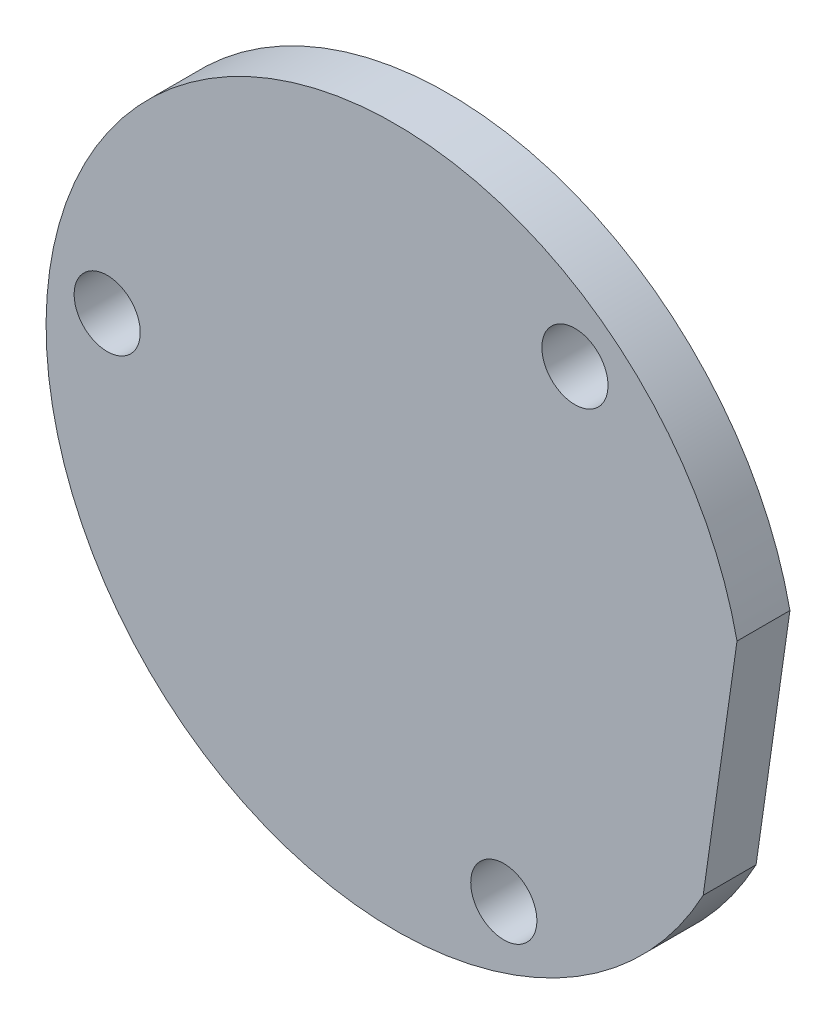
from build123d import *

# Parameters (mm, degrees)
BOSS_EXTRUDE1_DEPTH          = 10
SKETCH2_W                    = 45
SKETCH2_H                    = 4
F_12_5_12_5_DIAMETER_HOLE1_D = 12.5
M64_CLEARANCE_HOLE1_D        = 70
M64_CLEARANCE_HOLE1_DEPTH    = 4


with BuildPart() as part:
    # Sketch1 → Boss-Extrude1 (new body)
    with BuildSketch(Plane.XY.offset(-144.692981355)):
        with BuildLine():
            Line((511.459420647, 9.123067621), (517.84745191, 53.924775809))
            ThreePointArc((517.84745191, 53.924775809), (387.935069604, 49.592002612), (511.459420647, 9.123067621))
        make_face()
    extrude(amount=-BOSS_EXTRUDE1_DEPTH)

    # Sketch2 → Revolve1 (revolve)
    with BuildSketch(Plane(origin=(0, 40.2756484, 0), x_dir=(1, 0, 0), z_dir=(0, 1, 0))):
        with Locations((475.77422742, 156.692981355)):
            Rectangle(SKETCH2_W, SKETCH2_H)
    revolve(axis=Axis((453.27422742, 40.2756484, -158.692981355), (0, 0, 1)))

    # Ø12.5 (12.5) Diameter Hole1 (through all)
    with Locations(Plane(origin=(0, 0, -154.692981355), x_dir=(-1, 0, 0), z_dir=(0, 0, -1))):
        with Locations((-398.82492924, 48.03927691), (-487.222376026, 83.548309587), (-473.775376995, -10.760641298)):
            Hole(F_12_5_12_5_DIAMETER_HOLE1_D / 2)

    # M64 Clearance Hole1
    with Locations(Plane(origin=(0, 0, -158.692981355), x_dir=(-1, 0, 0), z_dir=(0, 0, -1))):
        with Locations((-453.27422742, 40.2756484)):
            Hole(M64_CLEARANCE_HOLE1_D / 2, depth=M64_CLEARANCE_HOLE1_DEPTH)


solid = part.part
